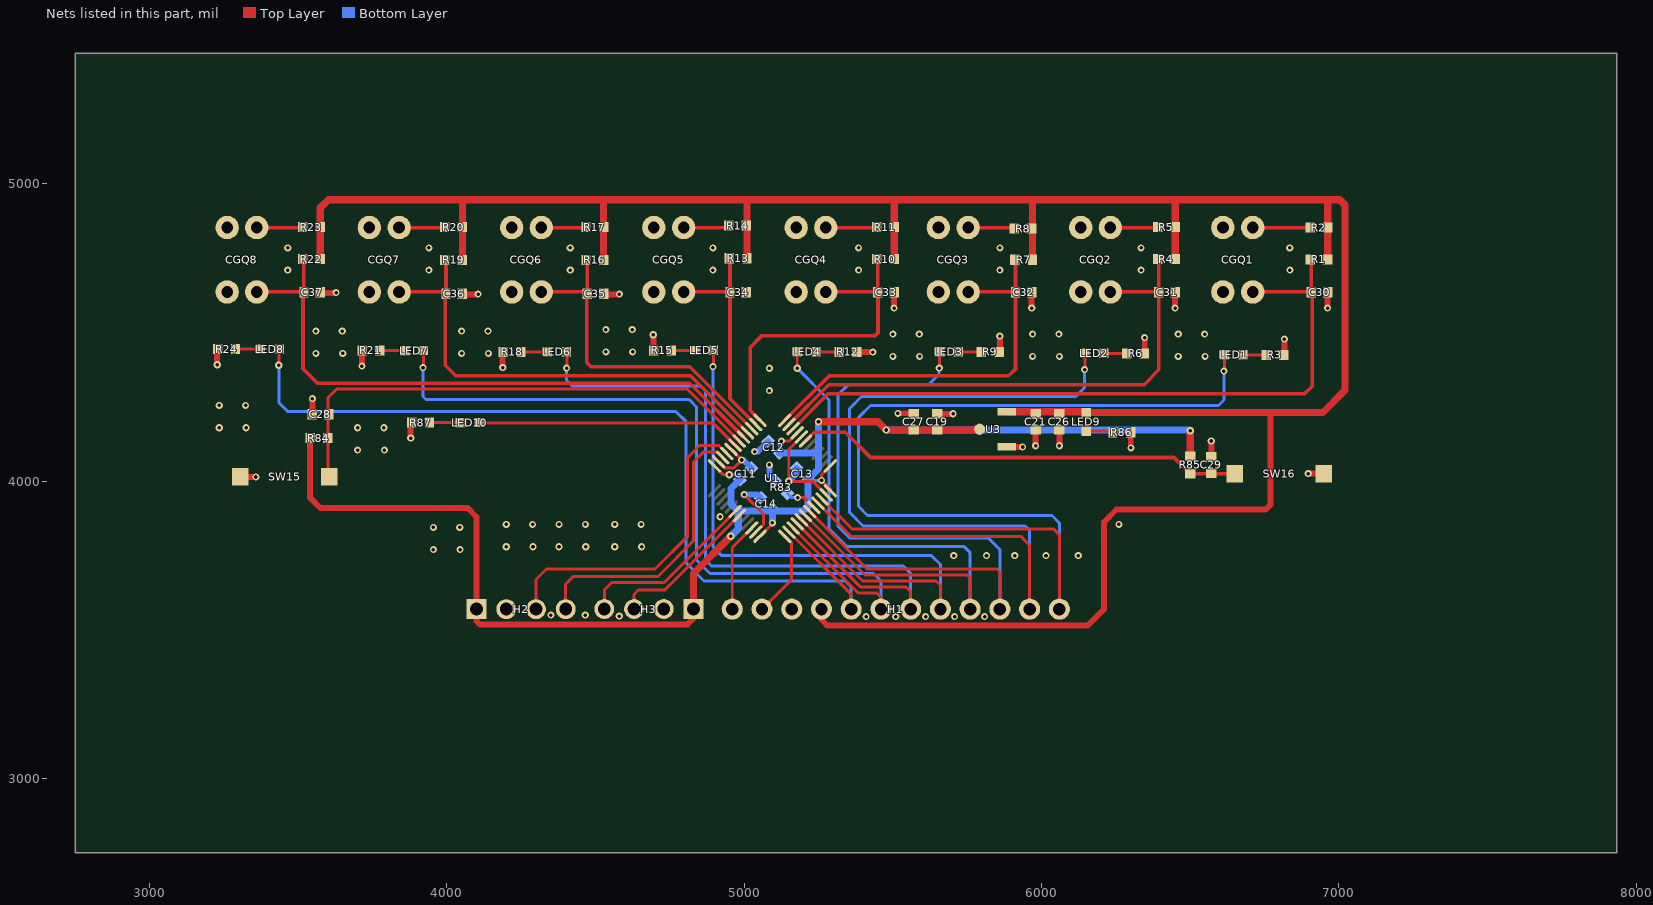
[diagram p0: the nets of this part, all layers, seen from the top]
# Altium PCB MISC51279.pcbdoc (part 2 of 3)
Units mil, origin at the board's own origin, x right, y up, seen from the top; angles counter-clockwise.
Board outline 5185 x 2690 mil, 2 copper layers (Top Layer, Bottom Layer), stack 62.206 mil thick; 72 components, 47 nets, 221 pads, 129 vias.

## Via types
v1: diameter 24.02, hole 12, Top Layer to Bottom Layer, 129 vias

## Nets (pads, with @x,y where several pads share a name; then routed paths per layer and width w, separated by ;. In a path a pad name is that pad's centre, name@x,y a point inside that pad or via, vN(x,y) a via of type N, cw(c..) or ccw(c..) an arc to the next point about the centre after c; other vN are vias at no path point)
3V3: C11.2 C12.2 C13.2 C14.2 C19.2 C27.1 H2.1 H3.1 R84.2 R85.2 U1.1 U1.9 U1.24 U1.36 U1.48 U3.2 | length 5218.3
  Top Layer w10: U1.24@4900.13,4051.75 4929.88,4022.01 v1(4950,4022.01) ; U1.36@5053.25,3815.13 5095,3856.88 v1(5095,3860) ; v1(5125.41,4135) 5150.41,4135 U1.9@5178.52,4163.11 ; U1.48@5289.87,3968.25 5289.87,3973.25 v1(5260,4003.12) 5260,4021.88 U1.1@5289.87,4051.75
  Top Layer w20: R84.2@3540.34,4145 3540.34,3944.66 3575,3910 4070,3910 4100,3880 H2.1@4100,3570 4100,3530 4111.18,3518.82 4809.69,3518.82 4829.69,3538.82 H3.1@4829.69,3570.18
  Top Layer w24: H3.1@4829.69,3570.18 4829.69,3689.69 v1(4955,3815) ; v1(5250,4200) 5450.3,4200 v1(5477.87,4172.43) C27.1@5570,4172.43 C19.2@5650,4172.43 5774.05,4172.43 U3.2@5776.61,4174.98 ; R85.2@6500,4084.66 v1(6500,4170)
  Bottom Layer w10: v1(4950,4022.01) 4969.02,4022.01 C11.2@4985.51,4005.51 ; C12.2@5119.49,4095.51 5119.49,4129.08 v1(5125.41,4135) ; C13.2@5214.49,4005.51 5216.88,4003.12 v1(5260,4003.12)
  Bottom Layer w24: v1(4955,3815) 4980,3840 4980,3900 ; C11.2@4985.51,4005.51 4956,3976 4956,3924 4980,3900 ; v1(5095,3860) C14.2@5095,3900 ; C12.2@5119.49,4095.51 5248.03,4095.51 5250,4093.55 ; v1(5250,4200) 5250,4093.55 ; v1(5477.87,4172.43) 6497.57,4172.43 v1(6500,4170) ; 4980,3900 C14.2@5095,3900 ; C14.2@5095,3900 5200,3900 5214.49,3914.49 C13.2@5214.49,4005.51 5250,4041.02 5250,4093.55
$1N696: LED1.1 R3.1 | length 77.7
  Top Layer w10: LED1.1@6677.75,4425.34 6755.29,4425.34 R3.1@6755.42,4425.21
$1N748: CGQ1.3 R2.1 | length 193.2
  Top Layer w12: CGQ1.3@6710,4853.3 6903.03,4853.3 R2.1@6903.15,4853.42
$1N1284: LED2.1 R6.1 | length 77.7
  Top Layer w10: LED2.1@6209.02,4430.34 6286.56,4430.34 R6.1@6286.7,4430.21
$1N1289: CGQ2.3 R5.1 | length 159.4
  Top Layer w12: CGQ2.3@6231.61,4853.3 6388.64,4853.3 R5.1@6390.34,4855
$1N1526: LED3.1 R9.1 | length 77.7
  Top Layer w10: LED3.1@5720.29,4435.34 5797.83,4435.34 R9.1@5797.97,4435.21
$1N1531: CGQ3.3 R8.1 | length 156.3
  Top Layer w12: CGQ3.3@5753.22,4853.3 5904.85,4853.3 R8.1@5908.15,4850
$1N2230: CGQ5.3 R14.1 | length 154.5
  Top Layer w12: CGQ5.3@4796.44,4853.3 4941.45,4853.3 R14.1@4948.15,4860
$1N2235: CGQ6.3 R17.1 | length 150.8
  Top Layer w12: CGQ6.3@4318.04,4853.3 4466.45,4853.3 R17.1@4468.15,4855
$1N2239: LED6.1 R18.1 | length 88.9
  Top Layer w10: R18.1@4249.66,4435 4338.38,4435 LED6.1@4338.52,4434.87
$1N2243: LED5.1 R15.1 | length 78.9
  Top Layer w10: R15.1@4754.66,4440 4833.38,4440 LED5.1@4833.52,4439.87
$1N2248: LED4.1 R12.1 | length 77.7
  Top Layer w10: LED4.1@5241.56,4435.34 5319.1,4435.34 R12.1@5319.24,4435.21
$1N2250: CGQ4.3 R11.1 | length 171.2
  Top Layer w12: CGQ4.3@5274.83,4853.3 5443.64,4853.3 R11.1@5445.34,4855
$1N2742: LED8.1 R24.1 | length 83.9
  Top Layer w10: R24.1@3289.49,4444.58 3373.22,4444.58 LED8.1@3373.35,4444.44
$1N2746: LED7.1 R21.1 | length 83.1
  Top Layer w10: R21.1@3774.66,4440 LED7.1@3857.8,4440
$1N2749: CGQ7.3 R20.1 | length 154.2
  Top Layer w12: CGQ7.3@3839.65,4853.3 3991.45,4853.3 R20.1@3993.15,4855
$1N2756: CGQ8.3 R23.1 | length 154.8
  Top Layer w12: CGQ8.3@3361.26,4853.3 3513.64,4853.3 R23.1@3515.34,4855
$1N3211: R83.2 U1.44 | length 107.5
  Top Layer w10: v1(5180,3945) 5201.76,3945 U1.44@5234.19,3912.57
  Bottom Layer w10: R83.2@5145.97,3959.03 5160,3945 v1(5180,3945)
$1N3907: LED9.1 R86.1 | length 91.7
  Top Layer w10: LED9.1@6150.13,4168.52 6236.82,4168.52 R86.1@6240.34,4165
$1N4007: LED10.1 R87.1 | length 103.7
  Top Layer w10: R87.1@3942,4197.24 LED10.1@4045.72,4197.24
ADC1: C30.1 CGQ1.1 R1.1 U1.10 | length 2431.8
  Top Layer w12: U1.10@5164.59,4177.03 5282.56,4295 6885,4295 6910,4320 6910,4632.44 C30.1@6907.44,4635 ; CGQ1.1@6710,4636.7 6905.74,4636.7 C30.1@6907.44,4635 ; R1.1@6903.15,4746.18 6907.44,4741.89 C30.1@6907.44,4635
ADC2: C31.1 CGQ2.1 R4.1 U1.11 | length 1857.9
  Top Layer w12: U1.11@5150.68,4190.95 5284.73,4325 6345,4325 6394.63,4374.63 C31.1@6394.63,4635 ; CGQ2.1@6231.61,4636.7 6392.93,4636.7 C31.1@6394.63,4635 ; R4.1@6390.34,4746.97 6394.63,4742.68 C31.1@6394.63,4635
ADC3: C32.1 CGQ3.1 R7.1 U1.12 | length 1375.5
  Top Layer w12: U1.12@5136.75,4204.87 5286.88,4355 5890,4355 5912.44,4377.44 C32.1@5912.44,4635 ; CGQ3.1@5753.22,4636.7 5910.74,4636.7 C32.1@5912.44,4635 ; R7.1@5910.34,4745 5912.44,4742.9 C32.1@5912.44,4635
ADC4: C33.1 CGQ4.1 R10.1 U1.13 | length 1134
  Top Layer w12: U1.13@5053.25,4204.87 5020,4238.12 5020,4450 5060,4490 5440,4490 5450,4500 5450,4634.63 C33.1@5449.63,4635 ; CGQ4.1@5274.83,4636.7 5447.93,4636.7 C33.1@5449.63,4635 ; R10.1@5445.34,4746.97 5449.63,4742.68 C33.1@5449.63,4635
ADC5: C34.1 CGQ5.1 R13.1 U1.14 | length 752.6
  Top Layer w12: CGQ5.1@4796.44,4636.7 4950.74,4636.7 C34.1@4952.44,4635 ; R13.1@4950.34,4750 4952.44,4747.9 C34.1@4952.44,4635 ; U1.14@5039.32,4190.95 4952.44,4277.83 C34.1@4952.44,4635
ADC6: C35.1 CGQ6.1 R16.1 U1.15 | length 1152.2
  Top Layer w12: CGQ6.1@4318.04,4636.7 4465.74,4636.7 C35.1@4472.44,4630 ; R16.1@4468.15,4744.47 4472.44,4740.18 C35.1@4472.44,4630 ; U1.15@5025.41,4177.03 4817.44,4385 4485,4385 4470,4400 4470,4627.56 C35.1@4472.44,4630
ADC7: C36.1 CGQ7.1 R19.1 U1.16 | length 1628.3
  Top Layer w12: CGQ7.1@3839.65,4636.7 3990.74,4636.7 C36.1@3997.44,4630 ; R19.1@3993.15,4744.47 3997.44,4740.18 C36.1@3997.44,4630 ; U1.16@5011.48,4163.11 4819.59,4355 4030,4355 3995,4390 3995,4627.56 C36.1@3997.44,4630
ADC8: C37.1 CGQ8.1 R22.1 U1.17 | length 2106.7
  Top Layer w12: CGQ8.1@3361.26,4636.7 3517.94,4636.7 C37.1@3519.63,4635 ; R22.1@3515.34,4746.97 3519.63,4742.68 C37.1@3519.63,4635 ; U1.17@4997.57,4149.19 4816.76,4330 3565,4330 3516.51,4378.49 3516.51,4631.88 C37.1@3519.63,4635
GND: C11.1 C12.1 C13.1 C14.1 C19.1 C21.1 C26.2 C27.2 C28.1 C29.1 C30.2 C31.2 C32.2 C33.2 C34.2 C35.2 C36.2 C37.2 CGQ1.2 CGQ1.4 CGQ2.2 CGQ2.4 CGQ3.2 CGQ3.4 CGQ4.2 CGQ4.4 CGQ5.2 CGQ5.4 CGQ6.2 CGQ6.4 CGQ7.2 CGQ7.4 CGQ8.2 CGQ8.4 H1.10 H2.2 H3.2 R3.2 R6.2 R9.2 R12.2 R15.2 R18.2 R21.2 R24.2 R83.1 R86.2 R87.2 SW15.2 SW16.2 U1.8 U1.20 U1.23 U1.35 U1.47 U3.1 | length 2216
  Top Layer w10: U1.23@4914.05,4065.68 4934.73,4045 4965,4045 v1(4991.62,4071.62) U1.20@4955.81,4107.43 ; v1(5000,3955) 5065,3890 5065,3854.73 U1.35@5039.32,3829.05 ; U1.8@5192.43,4149.19 5150,4106.76 v1(5150,4000) 5230.27,4000 U1.47@5275.95,3954.32
  Top Layer w20: v1@3227.35,4393.53 R24.2@3227.35,4443.98 ; SW15.2@3305.99,4013.81 v1@3356.45,4013.81 ; C28.1@3548.63,4225.59 v1@3548.63,4276.05 ; C37.2@3575.35,4633.82 v1@3625.81,4633.82 ; v1@3714.15,4388.95 R21.2@3714.15,4439.41 ; v1@3878.18,4146.98 R87.2@3878.18,4197.44 ; R87.2@3879.36,4198.03 R87.2@3879.63,4197.77 ; C36.2@4053.15,4628.81 v1@4103.61,4628.81 ; v1@4187.51,4383.95 R18.2@4187.51,4434.41 ; C35.2@4528.15,4628.81 v1@4578.61,4628.81 ; R15.2@4694.89,4440.59 v1@4694.89,4491.05 ; R12.2@5380.79,4434.02 v1@5431.25,4434.02 ; v1@5503.57,4583.95 C33.2@5503.57,4634.41 ; v1@5518.95,4228.74 C27.2@5569.41,4228.74 ; C19.1@5650.6,4226.36 v1@5701.06,4226.36 ; R9.2@5860.11,4435.8 v1@5860.11,4486.26 ; U3.1@5883.99,4114.75 v1@5934.45,4114.75 ; v1@5966.37,4583.95 C32.2@5966.37,4634.41 ; v1@5979.61,4121.38 C21.1@5979.61,4171.84 ; v1@6059.76,4121.38 C26.2@6059.76,4171.84 ; v1@6300.11,4113.95 R86.2@6300.11,4164.41 ; R6.2@6347.2,4430.8 v1@6347.2,4481.26 ; v1@6448.57,4583.95 C31.2@6448.57,4634.41 ; C29.1@6571.19,4083.15 v1@6571.19,4133.61 ; R3.2@6817.57,4425.8 v1@6817.57,4476.26 ; v1@6898.55,4026.19 SW16.2@6949.01,4026.19 ; v1@6961.37,4583.95 C30.2@6961.37,4634.41
  Bottom Layer w20: v1(4991.62,4071.62) 4997.36,4071.62 C11.1@5024.49,4044.49 ; v1(5000,3955) 5045,3955 C14.1@5055.51,3944.49 ; v1(5035,4100) 5046.02,4100 C12.1@5080.51,4134.49 ; v1(5085,4055) 5085,4020 R83.1@5104.03,4000.97 ; v1(5150,4000) 5175.51,4025.51 C13.1@5175.51,4044.49
  other v1: 5410,3545 5510,3545 5610.4,3545 5707.77,3545 5808.55,3545 4580,3546.81 4350,3550 4465.79,3550 5705,3750 5814.99,3750 5909.99,3750 6014.99,3750 6123.65,3750 3955,3770 4044.99,3770 4200,3780 4289.99,3780 4377.4,3780 4467.39,3780 4565,3780 4654.99,3780 3954.99,3845 4043.65,3845 4199.99,3855 4288.65,3855 4377.39,3855 4466.05,3855 4564.99,3855 4653.65,3855 6260,3855 4919.28,3880.72 3358.23,4014.41 6896.77,4025.59 3700,4105 3789.99,4105 6300.71,4112.17 5936.23,4115.34 5980.21,4119.6 6060.35,4119.6 6570.59,4135.39 3878.77,4145.2 3235,4180 3324.99,4180 3699.99,4180 3788.65,4180 5702.84,4226.96 5517.17,4228.14 3234.99,4255 3323.65,4255 3548.03,4277.83 5085,4305 5084.99,4380 4188.11,4382.17 3714.75,4387.17 3227.94,4391.74 5500,4420 5589.99,4420 5970,4420 6059.99,4420 6460,4420 6549.99,4420 3560,4430 3649.99,4430 4050,4430 4139.99,4430 4535.01,4435.21 4625,4435.21 5433.03,4434.62 6816.98,4478.04 6346.61,4483.04 5859.52,4488.04 4694.29,4492.83 5499.99,4495 5588.65,4495 5969.99,4495 6058.65,4495 6459.99,4495 6548.65,4495 3559.99,4505 3648.65,4505 4049.99,4505 4138.65,4505 4535,4510.21 4623.66,4510.21 5504.16,4582.17 5966.97,4582.17 6449.16,4582.17 6961.97,4582.17 4105.39,4629.41 4580.39,4629.41 3627.59,4634.41 3465,4710 3940,4710 4415,4710 4895,4710 5385,4710 5860,4710 6335,4710 6835,4710 3464.99,4785 3939.99,4785 4414.99,4785 4894.99,4785 5384.99,4785 5859.99,4785 6334.99,4785 6834.99,4785
KEY1: C28.2 R84.1 SW15.1 U1.18 | length 1735.4
  Top Layer w10: SW15.1@3604.6,4015 3600,4019.6 3600,4280 3630,4310 4808.92,4310 U1.18@4983.64,4135.27
LED1: LED10.2 U1.19 | length 894.4
  Top Layer w10: LED10.2@4106.48,4196.48 4894.61,4196.48 U1.19@4969.73,4121.36
OUT1: H1.1 LED1.2 U1.46 | length 3790.5
  Top Layer w10: U1.46@5262.03,3940.41 5362.44,3840 6040,3840 6060,3820 H1.1@6060,3570 ; v1(6613.5,4370.36) 6614.81,4371.67 LED1.2@6614.79,4425.07
  Bottom Layer w10: H1.1@6060,3570 6060,3860 6035,3885 5415,3885 5385,3915 5385,4215 5425,4255 6595,4255 6613.5,4273.5 v1(6613.5,4370.36)
OUT2: H1.2 LED2.2 U1.45 | length 3164.9
  Top Layer w10: U1.45@5248.11,3926.48 5359.59,3815 5930,3815 5960,3785 H1.2@5960,3570 ; v1(6144.75,4375.36) 6146.06,4376.67 LED2.2@6146.06,4430.07
  Bottom Layer w10: H1.2@5960,3570 5960,3835 5945,3850 5400,3850 5355,3895 5355,4245 5395,4285 6115,4285 6144.75,4314.75 v1(6144.75,4375.36)
OUT3: H1.3 LED3.2 U1.43 | length 2512.3
  Top Layer w10: U1.43@5220.27,3898.64 5413.92,3705 5850,3705 5860,3695 H1.3@5860,3570 ; v1(5656.02,4380.36) 5657.33,4381.67 LED3.2@5657.33,4435.07
  Bottom Layer w10: v1(5656.02,4380.36) 5656.02,4361.02 5620,4325 5350,4325 5315,4290 5315,3850 5355,3810 5820,3810 5860,3770 H1.3@5860,3570
OUT4: H1.4 LED4.2 U1.42 | length 2082.7
  Top Layer w10: v1(5178.65,4380) LED4.2@5178.6,4435.07 ; U1.42@5206.36,3884.73 5406.08,3685 5750,3685 5760,3675 H1.4@5760,3570
  Bottom Layer w10: v1(5178.65,4380) 5285,4273.65 5285,3840 5345,3780 5740,3780 5760,3760 H1.4@5760,3570
OUT5: H1.5 LED5.2 U1.41 | length 2239.5
  Top Layer w10: v1(4895.17,4385.42) 4896.48,4386.73 LED5.2@4896.48,4440.14 ; U1.41@5192.43,3870.81 5398.24,3665 5645,3665 5660,3650 H1.5@5660,3570
  Bottom Layer w10: v1(4895.17,4385.42) 4895.17,3779.83 4925,3750 5630,3750 5660,3720 H1.5@5660,3570
OUT6: H1.6 LED6.2 U1.40 | length 2511
  Top Layer w10: v1(4402.73,4380.4) 4404.04,4381.71 LED6.2@4404.04,4435.11 ; U1.40@5178.52,3856.89 5390.41,3645 5544.02,3645 5560,3629.02 H1.6@5560,3570
  Bottom Layer w10: v1(4402.73,4380.4) 4402.73,4340 4422.73,4320 4855,4320 4870,4305 4870,3735 4890,3715 5535,3715 5560,3690 H1.6@5560,3570
OUT7: H1.7 LED7.2 U1.39 | length 2778.1
  Top Layer w10: v1(3919.98,4382.44) 3921.29,4383.75 LED7.2@3921.29,4437.15 ; U1.39@5164.59,3842.97 5382.56,3625 5445,3625 5460,3610 H1.7@5460,3570
  Bottom Layer w10: v1(3919.98,4382.44) 3919.98,4285 3929.98,4275 4815,4275 4840,4250 4840,3735 4885,3690 5435,3690 5460,3665 H1.7@5460,3570
OUT8: H1.8 LED8.2 U1.38 | length 3061.1
  Top Layer w10: v1(3435,4390) 3436.31,4391.31 LED8.2@3436.31,4444.72 ; U1.38@5150.68,3829.05 5360,3619.73 H1.8@5360,3570
  Bottom Layer w10: v1(3435,4390) 3435,4265 3465,4235 4770,4235 4805,4200 4805,3725 4865,3665 5340,3665 5360,3645 H1.8@5360,3570
OUT_RX: H3.4 U1.30 | length 613.9
  Top Layer w10: H3.4@4529.69,3570.18 4529.69,3634.69 4555,3660 4731.08,3660 U1.30@4969.73,3898.64
OUT_TX: H3.3 U1.31 | length 513.2
  Top Layer w10: H3.3@4629.69,3570.18 4629.69,3619.69 4645,3635 4733.92,3635 U1.31@4983.64,3884.73
PB10: H2.3 U1.21 | length 1094.5
  Top Layer w10: H2.3@4300,3570 4300,3670 4335,3705 4700,3705 4810,3815 4810,4080 4850,4120 4915.41,4120 U1.21@4941.89,4093.52
PB11: H2.4 U1.22 | length 960.2
  Top Layer w10: H2.4@4400,3570 4400,3655 4425,3680 4710,3680 4830,3800 4830,4065 4864.1,4099.1 4908.46,4099.1 U1.22@4927.97,4079.59
RESET: C29.2 R85.1 SW16.1 U1.7 | length 1514.3
  Top Layer w12: U1.7@5206.36,4135.27 5236.08,4165 5340,4165 5425,4080 6445.34,4080 R85.1@6500,4025.34 6650.06,4025.34 SW16.1@6650.4,4025
SWCLK: H1.11 U1.37 | length 296.2
  Top Layer w10: H1.11@5060,3570 5160,3670 5160,3791.88 U1.37@5136.75,3815.13
SWDIO: H1.12 U1.34 | length 300.1
  Top Layer w10: H1.12@4960,3570 4960,3777.56 U1.34@5025.41,3842.97
VCC: C21.2 C26.1 H1.9 LED9.2 R1.2 R2.2 R4.2 R5.2 R7.2 R8.2 R10.2 R11.2 R13.2 R14.2 R16.2 R17.2 R19.2 R20.2 R22.2 R23.2 U3.3 | length 9042.4
  Top Layer w20: H1.9@5260,3570 5260,3535 5280,3515 6155,3515 6210,3570 6210,3862.74 6252.26,3905 6753.87,3905 6770,3921.13 6770,4230
  Top Layer w24: R22.2@3574.66,4746.97 R23.2@3574.66,4855 3574.66,4919.66 3601.97,4946.97 4054.84,4946.97 ; R19.2@4052.47,4744.47 R20.2@4052.47,4855 4052.47,4944.59 4054.84,4946.97 ; R16.2@4527.47,4744.47 R17.2@4527.47,4855 4527.47,4945.87 4528.57,4946.97 ; R13.2@5009.66,4750 5009.66,4942.27 5004.96,4946.97 ; R10.2@5504.66,4746.97 R11.2@5504.66,4855 5504.66,4946.23 5505.4,4946.97 ; U3.3@5883.4,4234.05 6147.3,4234.05 LED9.2@6149.86,4231.48 6946.48,4231.48 7020,4305 7020,4930 7003.03,4946.97 6964.56,4946.97 ; R7.2@5969.66,4745 5969.66,4943.97 5966.66,4946.97 ; R4.2@6449.66,4746.97 R5.2@6449.66,4855 6449.66,4945.7 6448.39,4946.97 ; R1.2@6962.47,4746.18 R2.2@6962.47,4853.42 6962.47,4944.87 6964.56,4946.97 ; 4054.84,4946.97 4528.57,4946.97 ; 4528.57,4946.97 5004.96,4946.97 ; 5004.96,4946.97 5505.4,4946.97 ; 5505.4,4946.97 5966.66,4946.97 ; 5966.66,4946.97 6448.39,4946.97 ; 6448.39,4946.97 6964.56,4946.97
pads on no net: U1.2 U1.3 U1.4 U1.5 U1.6 U1.25 U1.26 U1.27 U1.28 U1.29 U1.32 U1.33

## Polygon pours and split planes (outlines as drawn)
GND on Bottom Layer (solid, remove dead copper, pour order 2): 3070,5170 3070,3005 7685,3005 7685,5170
GND on Top Layer (solid, remove dead copper, pour order 0): 3000,5190 3000,3000 7550,3000 7550,5190

## Keep-outs
Board Outline Layer:
  region: 3850.31,4056.06 ccw(c3850.31,3995.04) 3789.29,3995.04 ccw(c3850.31,3995.04) 3850.31,3934.02 4712.52,3934.02 ccw(c4712.52,3995.04) 4773.54,3995.04 ccw(c4712.52,3995.04) 4712.52,4056.06 3850.31,4056.06
  region: 3850.31,4056.06 ccw(c3850.31,3995.04) 3789.29,3995.04 ccw(c3850.31,3995.04) 3850.31,3934.02 4712.52,3934.02 ccw(c4712.52,3995.04) 4773.54,3995.04 ccw(c4712.52,3995.04) 4712.52,4056.06 3850.31,4056.06
  region: 5464.49,4056.06 ccw(c5464.49,3995.04) 5403.46,3995.04 ccw(c5464.49,3995.04) 5464.49,3934.02 6326.69,3934.02 ccw(c6326.69,3995.04) 6387.72,3995.04 ccw(c6326.69,3995.04) 6326.69,4056.06 5464.49,4056.06
  region: 5464.49,4056.06 ccw(c5464.49,3995.04) 5403.46,3995.04 ccw(c5464.49,3995.04) 5464.49,3934.02 6326.69,3934.02 ccw(c6326.69,3995.04) 6387.72,3995.04 ccw(c6326.69,3995.04) 6326.69,4056.06 5464.49,4056.06
  lines w0.1: 3789.29,3995.04 cw(c3850.31,3995.04) 3850.31,4056.06 4712.52,4056.06 cw(c4712.52,3995.04) 4773.54,3995.04 cw(c4712.52,3995.04) 4712.52,3934.02 3850.31,3934.02 cw(c3850.31,3995.04) 3789.29,3995.04 ; 5403.46,3995.04 cw(c5464.49,3995.04) 5464.49,4056.06 6326.69,4056.06 cw(c6326.69,3995.04) 6387.72,3995.04 cw(c6326.69,3995.04) 6326.69,3934.02 5464.49,3934.02 cw(c5464.49,3995.04) 5403.46,3995.04
  lines w3.94: 3121.5,3996.81 ccw(c3239.61,3996.81) 3239.61,3878.7 3790.79,3878.7 cw(c3790.79,3760.59) 3908.9,3760.59 3908.9,3603.11 ccw(c4027.01,3603.11) 4027.01,3485 6152.99,3485 ccw(c6152.99,3603.11) 6271.1,3603.11 6271.1,3760.59 cw(c6389.21,3760.59) 6389.21,3878.7 6940.39,3878.7 ccw(c6940.39,3996.81) 7058.5,3996.81 7058.5,4941.69 ccw(c6940.39,4941.69) 6940.39,5059.8 3239.61,5059.8 ccw(c3239.61,4941.69) 3121.5,4941.69 3121.5,3996.81

## Other copper
Top Layer:
  drawing of 238 lines, arcs and shapes, not listed